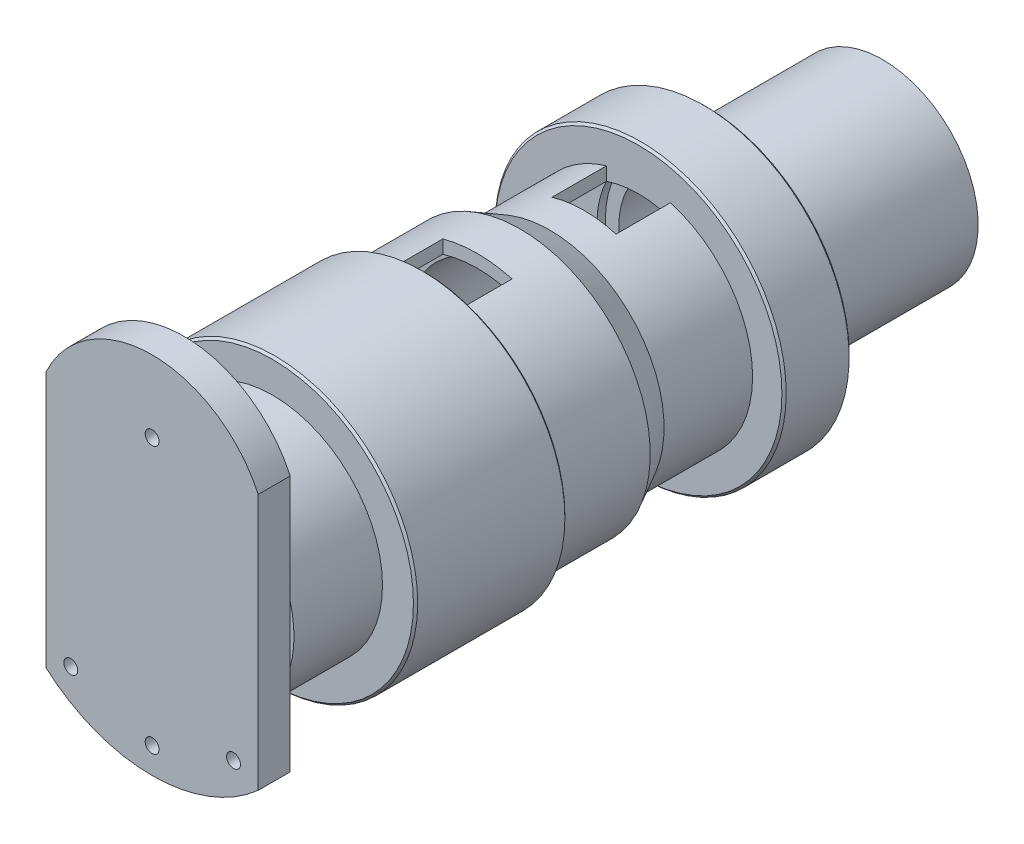
SolidWorks part; units mm, degrees
ref_plane "前视基准面" through (0, 0, 0) normal (0, 0, 1) x (1, 0, 0)
ref_plane "上视基准面" through (0, 0, 0) normal (0, 1, 0) x (1, 0, 0)
ref_plane "右视基准面" through (0, 0, 0) normal (1, 0, 0) x (0, 0, -1)
other "Configuration Table"
sketch "草图2" plane through (0, 0, 0) normal (0, 0, 1) x (1, 0, 0)
  line L0 (0, 347.7728) -> (0, -240.8779) construction
  line L1 (-107.5, 21.352) -> (-107.5, -186.718)
  line L2 (107.5, 21.352) -> (107.5, -186.718)
  arc A0 (107.5, 21.352) -> (-107.5, 21.352) centre (0, 0) ccw
  arc A1 (-107.5, -186.718) -> (107.5, -186.718) centre (0, -82.1056) ccw
  point P12 (107.5, -82.683)
  dimension "D1" = 300
  dimension "D2" = 219.2
  dimension "D4" = 215
  dimension "D3" = 208.07
extrude "凸台-拉伸1" add sketch "草图2" along normal blind 30
sketch "草图3" plane through (0, 0, 0) normal (0, 0, -1) x (-1, 0, 0)
  line L0 (0, 218.8134) -> (0, -307.4921) construction
  line L1 (-107.5, -82.683) -> (107.5, -82.683) construction
  line L2 (-107.5, -186.718) -> (-107.5, 21.352) construction
  line L3 (107.5, 21.352) -> (107.5, -186.718) construction
  circle A0 centre (0, -82.683) radius 93
  circle A1 centre (0, -82.683) radius 103
  dimension "D1" = 186
  dimension "D2" = 206
extrude "凸台-拉伸2" add sketch "草图3" along normal blind 85
ref_axis "基准轴1" through (0, -82.683, -1172.4502) along (0, 0, 1)
ref_plane "基准面1" through (0, -82.683, 0) normal (0, 1, 0) x (0, 0, 1)
sketch "草图4" plane through (0, -82.683, 0) normal (0, 1, 0) x (0, 0, 1)
  line L0 (-95, -93) -> (-95, -122)
  line L1 (-95, -122) -> (-213, -122)
  line L2 (-213, -122) -> (-213, -110)
  line L3 (-213, -110) -> (-303, -110)
  line L4 (-303, -110) -> (-303, -95)
  line L5 (-303, -95) -> (-438, -95)
  line L6 (-83, -93) -> (-83, -134)
  line L7 (-83, -134) -> (-225, -134)
  line L8 (-438, -95) -> (-438, -124.5)
  line L9 (-438, -124.5) -> (-477, -124.5)
  line L10 (-477, -124.5) -> (-477, -90)
  line L11 (-477, -90) -> (-485, -90)
  line L12 (-485, -90) -> (-485, -77.5)
  line L13 (-485, -77.5) -> (-655, -77.5)
  line L14 (-85, 103) -> (-85, -103) construction
  line L15 (-1172.4502, 0) -> (521.6257, 0) construction
  line L16 (-225, -134) -> (-225, -122)
  line L17 (-225, -122) -> (-315, -122)
  line L19 (-343, -107) -> (-426, -107)
  line L20 (-426, -107) -> (-426, -136.5)
  line L21 (-426, -136.5) -> (-489, -136.5)
  line L25 (-497, -89.5) -> (-655, -89.5)
  line L26 (-95, -93) -> (-83, -93)
  line L27 (-655, -77.5) -> (-655, -89.5)
  line L28 (-497, -89.5) -> (-489, -136.5)
  line L29 (-489, -102) -> (-497, -102) construction
  line L30 (-497, -102) -> (-497, -89.5) construction
  line L31 (-489, -136.5) -> (-489, -102) construction
  line L32 (-315, -122) -> (-343, -107)
  line L33 (-315, -107) -> (-426, -107) construction
  line L34 (-315, -122) -> (-315, -107) construction
  dimension "D1" = 10
  dimension "D2" = 93
  dimension "D3" = 122
  dimension "D4" = 118
  dimension "D5" = 110
  dimension "D6" = 90
  dimension "D7" = 95
  dimension "D8" = 135
  dimension "D9" = 39
  dimension "D10" = 124.5
  dimension "D11" = 90
  dimension "D12" = 77.5
  dimension "D13" = 8
  dimension "D14" = 170
  dimension "D16" = 40
  dimension "D15" = 12
revolve "旋转1" add sketch "草图4" angle 360 about axis through (0, -82.683, -1172.4502) along (0, 0, 1)
chamfer "倒角1" distance 2 angle 45 1 edges at (-136.5, -82.683, -489)
chamfer "倒角2" distance 2 angle 45 3 edges at (-134, -82.683, -83) (-134, -82.683, -225) (-136.5, -82.683, -426)
sketch "草图5" plane through (0, -82.683, 0) normal (0, 1, 0) x (0, 0, 1)
  line L0 (-1172.4502, 0) -> (521.6257, 0) construction
  line L1 (-275, 32.5) -> (-225, 32.5)
  line L2 (-275, 32.5) -> (-275, -32.5)
  line L3 (-275, -32.5) -> (-225, -32.5)
  line L4 (-225, 32.5) -> (-225, -32.5)
  line L5 (-275, 32.5) -> (-225, -32.5) construction
  line L6 (-275, -32.5) -> (-225, 32.5) construction
  line L7 (-225, 122) -> (-225, -122) construction
  line L8 (-426, 30) -> (-375, 30)
  line L9 (-426, 30) -> (-426, -30)
  line L10 (-426, -30) -> (-375, -30)
  line L11 (-375, 30) -> (-375, -30)
  line L12 (-426, 30) -> (-375, -30) construction
  line L13 (-426, -30) -> (-375, 30) construction
  line L14 (-426, -107) -> (-426, 107) construction
  point P0 (-250, 0)
  point P7 (-400.5, 0)
  dimension "D1" = 0
  dimension "D2" = 65
  dimension "D3" = 50
  dimension "D4" = 0
  dimension "D5" = 60
  dimension "D6" = 51
extrude "切除-拉伸1" cut sketch "草图5" along normal blind 145
sketch "草图6" plane through (0, 0, 30) normal (0, 0, 1) x (1, 0, 0)
  line L0 (0, 280.942) -> (0, -407.3001) construction
  line L1 (-76.3151, -181.683) -> (76.3151, -181.683) construction
  circle A0 centre (0, -82.683) radius 125 construction
  circle A1 centre (0, 42.317) radius 6.5
  circle A2 centre (0, -207.683) radius 6.5
  circle A3 centre (-76.3151, -181.683) radius 6.5
  circle A4 centre (76.3151, -181.683) radius 6.5
  dimension "D1" = 250
  dimension "D2" = 13
  dimension "D3" = 13
  dimension "D4" = 13
  dimension "D5" = 13
  dimension "D6" = 26
extrude "切除-拉伸2" cut sketch "草图6" against normal up to next
sketch "草图7" plane through (0, 0, 30) normal (0, 0, 1) x (1, 0, 0)
  line L0 (-107.5, 21.352) -> (-107.5, -186.718) construction
  line L1 (-99.5, 62.5931) -> (-107.5, 62.5931)
  line L2 (-99.5, 62.5931) -> (-99.5, -227.9591)
  line L3 (-99.5, -227.9591) -> (-107.5, -227.9591)
  line L4 (-107.5, 62.5931) -> (-107.5, -227.9591)
  line L5 (-99.5, 62.5931) -> (-107.5, -227.9591) construction
  line L6 (-99.5, -227.9591) -> (-107.5, 62.5931) construction
  line L7 (107.5, -186.718) -> (107.5, 21.352) construction
  line L8 (99.5, 62.1963) -> (107.5, 62.1963)
  line L9 (99.5, 62.1963) -> (99.5, -227.5622)
  line L10 (99.5, -227.5622) -> (107.5, -227.5622)
  line L11 (107.5, 62.1963) -> (107.5, -227.5622)
  line L12 (99.5, 62.1963) -> (107.5, -227.5622) construction
  line L13 (99.5, -227.5622) -> (107.5, 62.1963) construction
  point P0 (-103.5, -82.683)
  point P7 (103.5, -82.683)
  dimension "D1" = 199
  dimension "D2" = 8
extrude "切除-拉伸3" cut sketch "草图7" against normal up to surface (30 mm away) up to face at (6.5, 42.317, 0)
